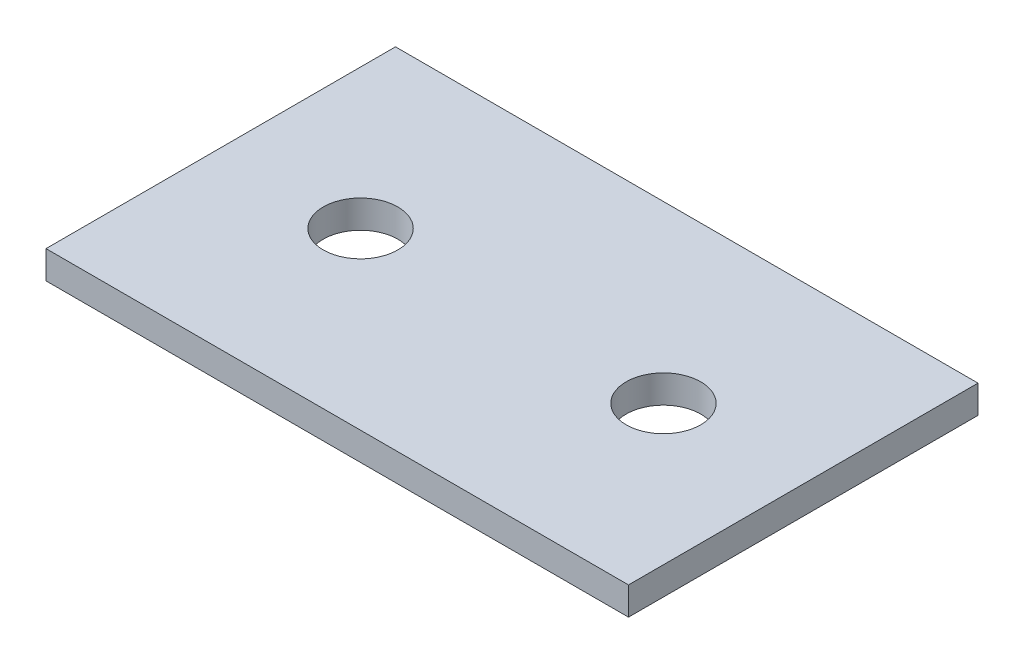
from build123d import *

# Parameters (mm, degrees)
SKETCH_1_W          = 250
SKETCH_1_H          = 150
EXTRUDE_1_DEPTH     = 12
SKETCH_2_R          = 10
CUT_EXTRUDE_1_DEPTH = 2
CUT_EXTRUDE_2_REACH = 148.267
SKETCH_3_R          = 16


with BuildPart() as part:
    # 草图1 → 凸台-拉伸1 (new body)
    with BuildSketch(Plane(origin=(0, 0, 0), x_dir=(1, 0, 0), z_dir=(0, 1, 0))):
        Rectangle(SKETCH_1_W, SKETCH_1_H)
    extrude(amount=EXTRUDE_1_DEPTH)

    # 草图2 → 切除-拉伸1 (cut)
    with BuildSketch(Plane(origin=(0, 0, 0), x_dir=(-1, 0, 0), z_dir=(0, -1, 0))):
        with Locations(Location((-108, 58, 0), (0, 0, 90))):
            Circle(SKETCH_2_R)
        with Locations(Location((108, 58, 0), (0, 0, 90))):
            Circle(SKETCH_2_R)
        with Locations(Location((-108, -58, 0), (0, 0, 90))):
            Circle(SKETCH_2_R)
        with Locations(Location((108, -58, 0), (0, 0, 90))):
            Circle(SKETCH_2_R)
    extrude(amount=-CUT_EXTRUDE_1_DEPTH, mode=Mode.SUBTRACT)

    # 草图3 → 切除-拉伸2 (cut, up to next)
    with BuildSketch(Plane(origin=(0, 12, 0), x_dir=(1, 0, 0), z_dir=(0, 1, 0)), mode=Mode.PRIVATE) as cut_extrude_2_sk1:
        with Locations(Location((-65, 0, 0), (0, 0, 270))):
            Circle(SKETCH_3_R)
    cut_extrude_2_tool1 = extrude(cut_extrude_2_sk1.sketch, amount=-CUT_EXTRUDE_2_REACH, mode=Mode.PRIVATE) & part.part
    # 草图3 → 切除-拉伸2 (cut, up to next)
    with BuildSketch(Plane(origin=(0, 12, 0), x_dir=(1, 0, 0), z_dir=(0, 1, 0)), mode=Mode.PRIVATE) as cut_extrude_2_sk2:
        with Locations(Location((65, 0, 0), (0, 0, 270))):
            Circle(SKETCH_3_R)
    cut_extrude_2_tool2 = extrude(cut_extrude_2_sk2.sketch, amount=-CUT_EXTRUDE_2_REACH, mode=Mode.PRIVATE) & part.part
    add(cut_extrude_2_tool1.solids().sort_by_distance((-65, 12, 0))[0], mode=Mode.SUBTRACT)
    add(cut_extrude_2_tool2.solids().sort_by_distance((65, 12, 0))[0], mode=Mode.SUBTRACT)


solid = part.part
